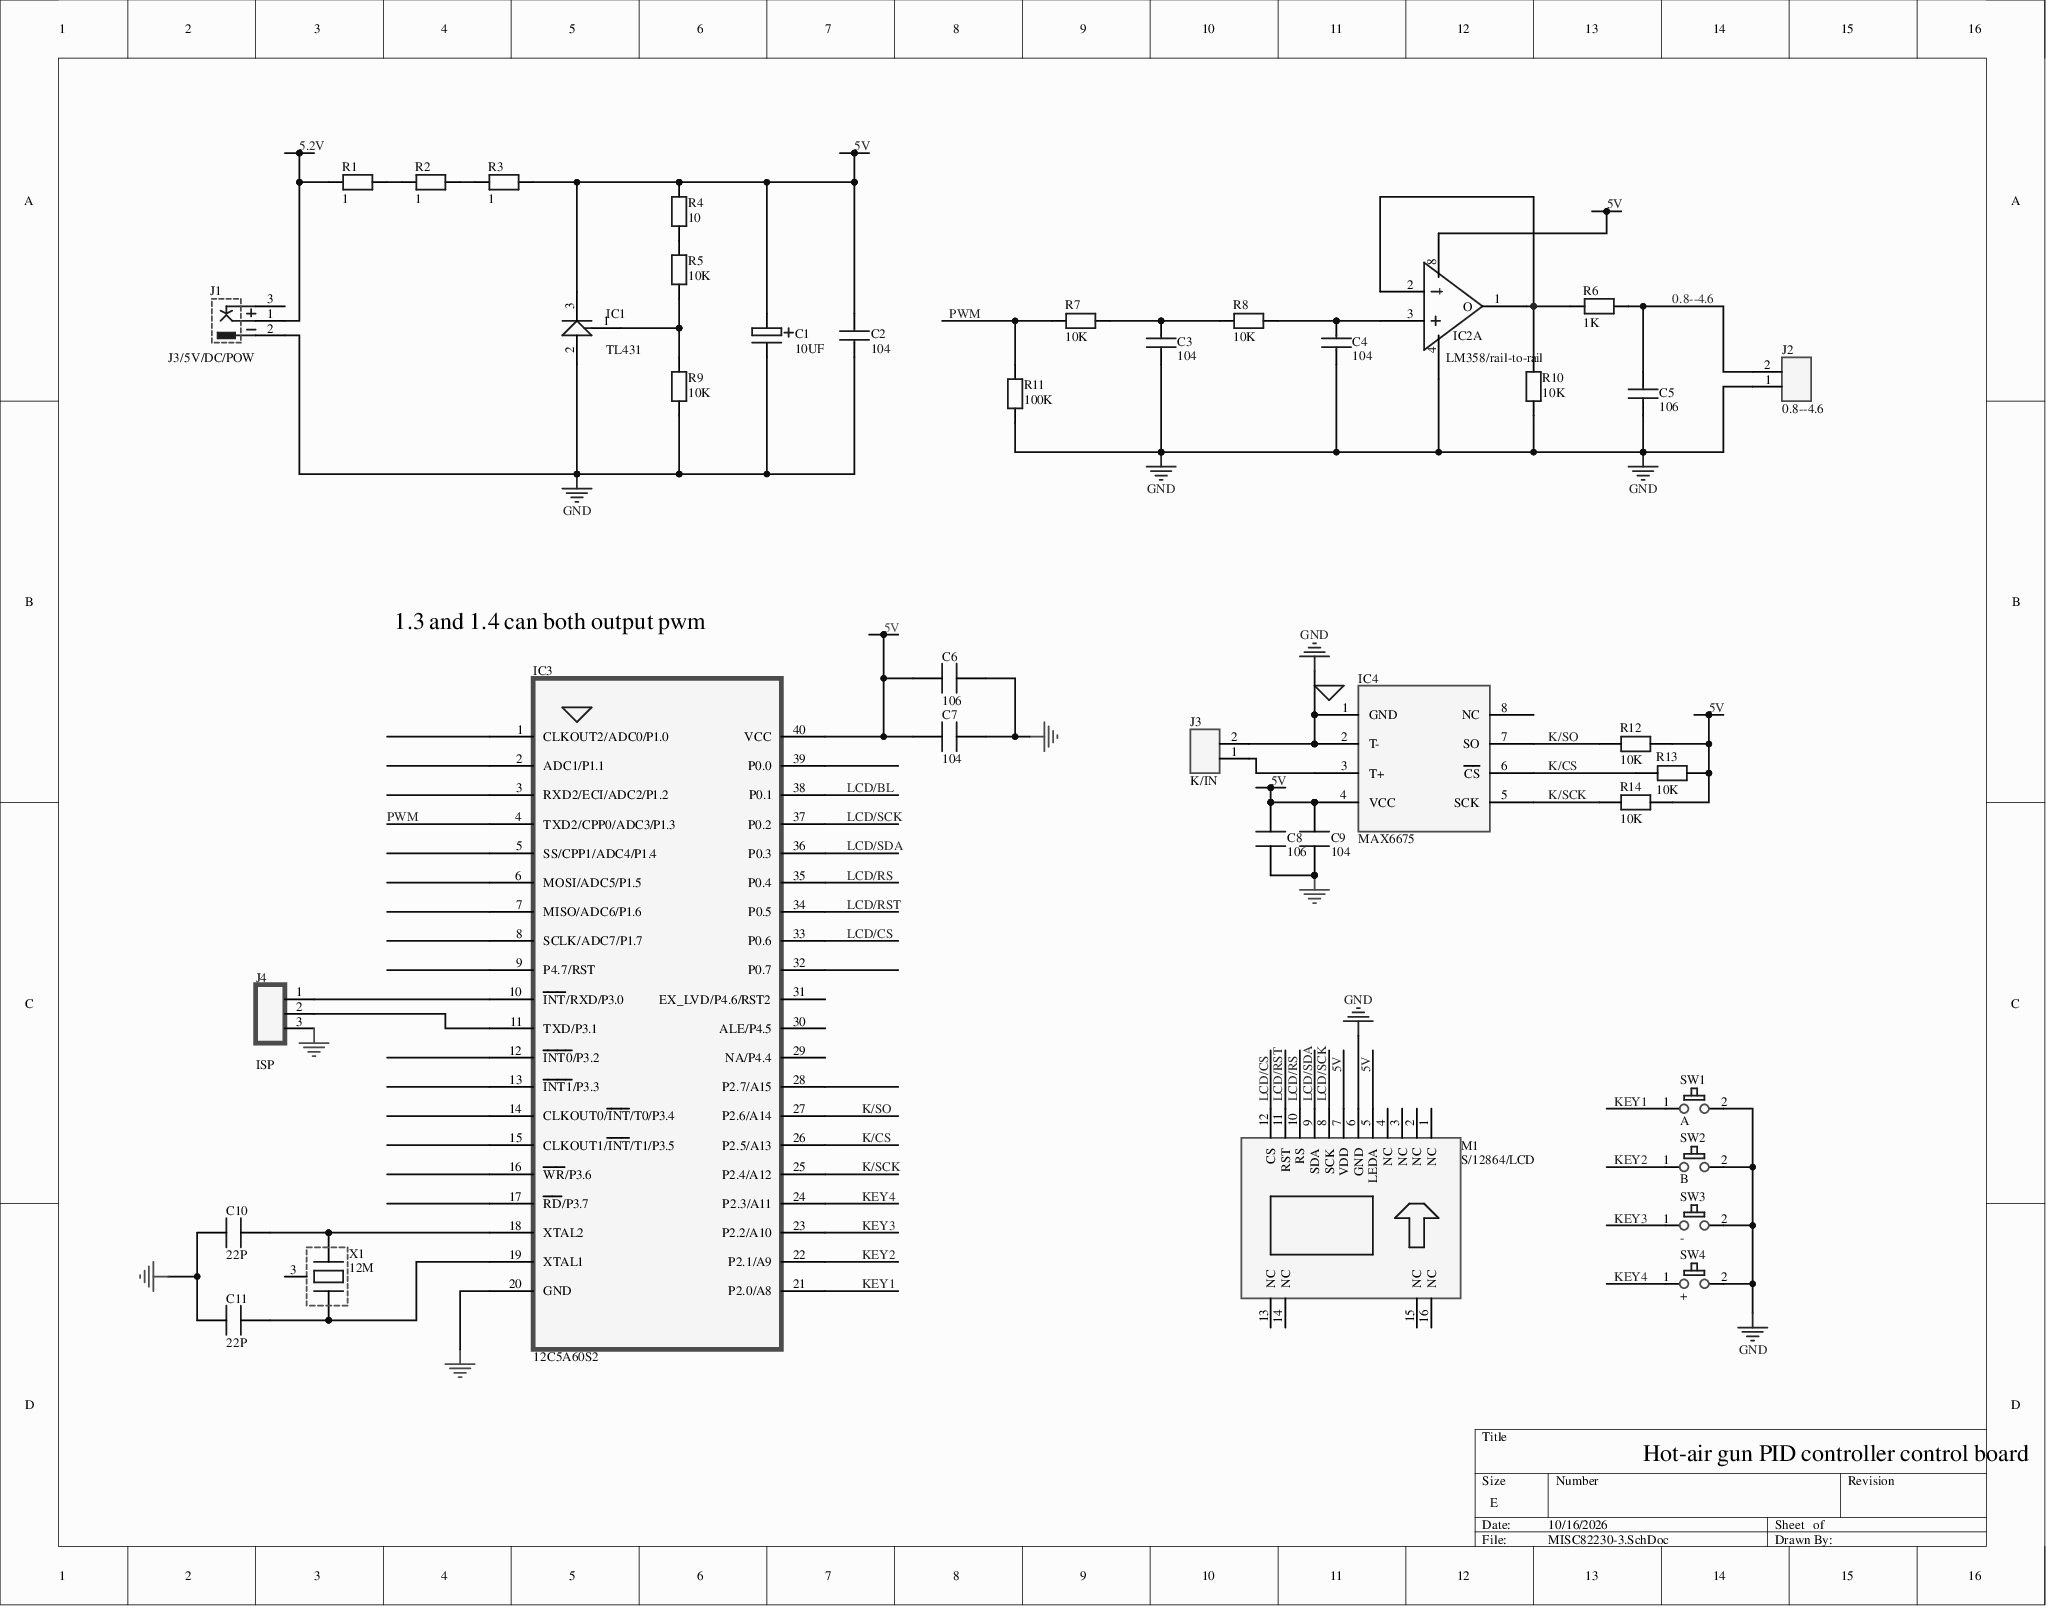
[diagram p0: MISC82230-3.SchDoc]
# Altium project MISC82230-2.PrjPcb
1 sheet, 39 parts. Net scope: global (net labels, ports and power ports of the same name join across sheets).
Board file: MISC82230.PcbDoc

## Sheet MISC82230-3.SchDoc
size 355 x 279 mm

### Parts
C1  10UF  [C10]
C2  104  [0805]
C3  104  [0805]
C4  104  [0805]
C5  106  [0805]
C6  106  [0805]
C7  104  [0805]
C8  106  [0805]
C9  104  [0805]
C10  22P  [0805]
C11  22P  [0805]
IC1  TL431  [TO92]
IC2  LM358/rail-to-rail  [SOP8]  (part A of 2)
IC3  12C5A60S2  [DIP40]
IC4  MAX6675  [SOP8]
J1  J3/5V/DC/POW  [DC/POW]
J2  0.8--4.6  [SIP2/8.5]
J3  K/IN  [SIP2/8.5]
J4  ISP  [SIP3]
M1  S/12864/LCD  [S/12864/LCD]
R1  1  [0805]
R2  1  [0805]
R3  1  [0805]
R4  10  [0805]
R5  10K  [0805]
R6  1K  [0805]
R7  10K  [0805]
R8  10K  [0805]
R9  10K  [0805]
R10  10K  [0805]
R11  100K  [0805]
R12  10K  [0805]
R13  10K  [0805]
R14  10K  [0805]
SW1  A  [BUTTON/B]
SW2  B  [BUTTON/B]
SW3  -  [BUTTON/B]
SW4  +  [BUTTON/B]
X1  12M  [X]

### Nets
GND: C1.2 C2.2 C3.2 C4.2 C5.2 C6.2 C7.2 C8.2 C9.2 C10.2 C11.2 IC1.2 IC2.4 IC3.20(GND) IC4.1(GND) IC4.2(T-) J1.2 J2.1 J3.2 J4.3 M1.6(GND) R9.2 R10.1 R11.1 SW1.2 SW2.2 SW3.2 SW4.2
0.8--4.6: C5.1 J2.2 R6.2
5.2V: J1.1(+) R1.2
5V: C1.1 C2.1 C6.1 C7.1 C8.1 C9.1 IC1.3 IC2.8(+) IC3.40(VCC) IC4.4(VCC) M1.5(LEDA) M1.7(VDD) R3.1 R4.1 R12.1 R13.1 R14.1
K/CS: IC3.26(P2.5/A13) IC4.6(~{CS}) R13.2
K/SCK: IC3.25(P2.4/A12) IC4.5(SCK) R14.2
K/SO: IC3.27(P2.6/A14) IC4.7(SO) R12.2
KEY1: IC3.21(P2.0/A8) SW1.1
KEY2: IC3.22(P2.1/A9) SW2.1
KEY3: IC3.23(P2.2/A10) SW3.1
KEY4: IC3.24(P2.3/A11) SW4.1
LCD/BL: IC3.38(P0.1)
LCD/CS: IC3.33(P0.6) M1.12(CS)
LCD/RS: IC3.35(P0.4) M1.10(RS)
LCD/RST: IC3.34(P0.5) M1.11(RST)
LCD/SCK: IC3.37(P0.2) M1.8(SCK)
LCD/SDA: IC3.36(P0.3) M1.9(SDA)
PWM: IC3.4(TXD2/CPP0/ADC3/P1.3) R7.1 R11.2
NetC3_1: C3.1 R7.2 R8.1
NetC4_1: C4.1 IC2.3 R8.2
NetC10_1: C10.1 IC3.18(XTAL2) X1.1
NetC11_1: C11.1 IC3.19(XTAL1) X1.2
NetIC1_1: IC1.1 R5.2 R9.1
NetIC2_1: IC2.1(O) IC2.2 R6.1 R10.2
NetIC3_10: IC3.10(~{INT}/RXD/P3.0) J4.1
NetIC3_11: IC3.11(TXD/P3.1) J4.2
NetIC4_3: IC4.3(T+) J3.1
NetR1_1: R1.1 R2.2
NetR2_1: R2.1 R3.2
NetR4_2: R4.2 R5.1

Not connected (* = marked no-connect by the designer): IC3 1(CLKOUT2/ADC0/P1.0)* 2(ADC1/P1.1)* 3(RXD2/ECI/ADC2/P1.2)* 5(SS/CPP1/ADC4/P1.4)* 6(MOSI/ADC5/P1.5)* 7(MISO/ADC6/P1.6)* 8(SCLK/ADC7/P1.7)* 9(P4.7/RST)* 12(~{INT0}/P3.2)* 13(~{INT1}/P3.3)* 14(CLKOUT0/~{INT}/T0/P3.4)* 15(CLKOUT1/~{INT}/T1/P3.5)* 16(~{WR}/P3.6)* 17(~{RD}/P3.7)* 28(P2.7/A15)* 29(NA/P4.4)* 30(ALE/P4.5)* 31(EX_LVD/P4.6/RST2)* 32(P0.7)* 39(P0.0)*; IC4 8(NC)*; J1 3*; M1 1(NC)* 2(NC)* 3(NC)* 4(NC)* 13(NC)* 14(NC)* 15(NC)* 16(NC)*; X1 3*

### Notes on the sheet
- 1.3 and 1.4 can both output pwm
- Hot-air gun PID controller control board

### Library data of the parts
C1 = CE
C2-C11 = C
IC2 = LM358
IC3 = 12C5A08AD
J2 J3 = J2
J4 = J3
R1-R14 = R
SW1-SW4 = SW2
X1 = X